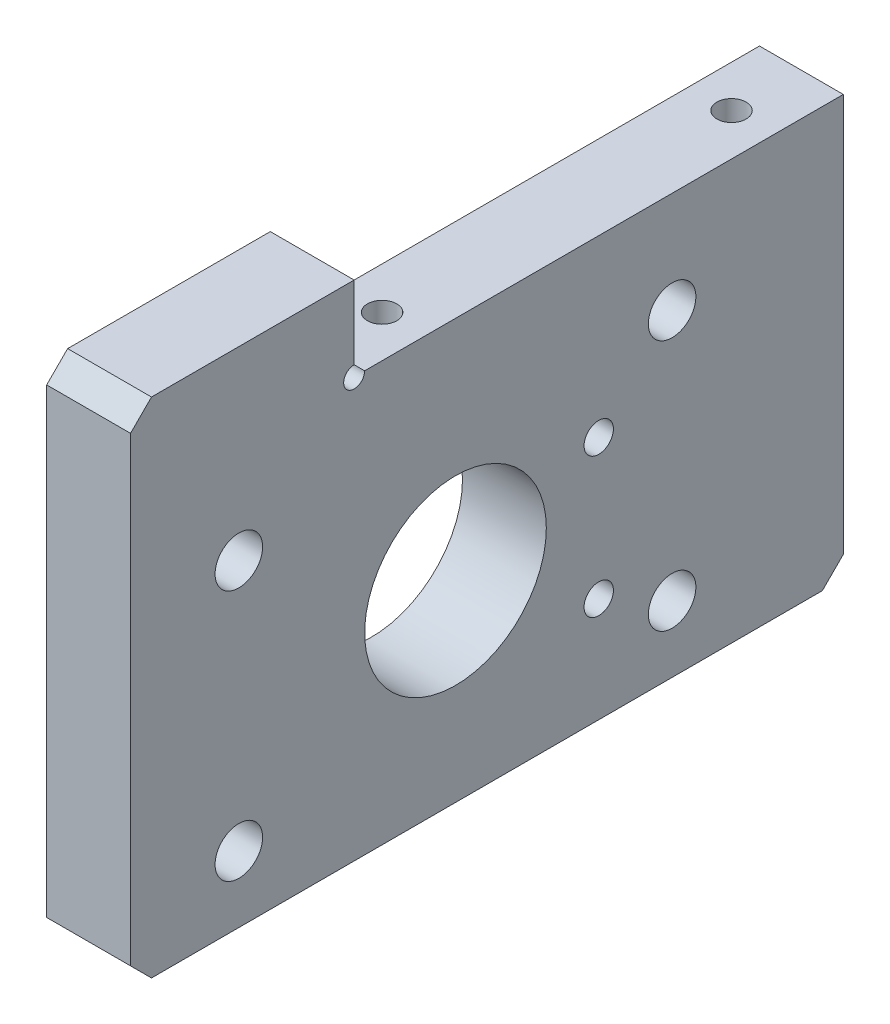
from build123d import *

# Parameters (mm, degrees)
BOSS_EXTRUDE1_DEPTH   = 12
SKETCH2_R             = 13
CUT_EXTRUDE1_DEPTH    = 126.427269762
M8_TAPPED_HOLE1_D     = 6.8
M8_TAPPED_HOLE1_DEPTH = 19.75
M8_TAPPED_HOLE1_TIP   = 2.042926105
M5_TAPPED_HOLE1_D     = 4.2
M5_TAPPED_HOLE1_DEPTH = 12.4
M5_TAPPED_HOLE1_TIP   = 1.2618073
M5_TAPPED_HOLE2_D     = 4.2
M5_TAPPED_HOLE2_DEPTH = 12.4
M5_TAPPED_HOLE2_TIP   = 1.2618073
CHAMFER1_SIZE         = 3
SKETCH11_R            = 1.5
CUT_EXTRUDE2_DEPTH    = 126.427269762


with BuildPart() as part:
    # Sketch1 → Boss-Extrude1 (new body)
    with BuildSketch(Plane(origin=(0, 0, 0), x_dir=(0, 0, -1), z_dir=(1, 0, 0))):
        Polygon((0, 0), (102, 0), (102, 60), (32, 60), (32, 72), (0, 72), align=None)
    extrude(amount=BOSS_EXTRUDE1_DEPTH)

    # Sketch2 → Cut-Extrude1 (cut, through all)
    with BuildSketch(Plane(origin=(12, 0, 0), x_dir=(0, 0, -1), z_dir=(1, 0, 0))):
        with Locations((46.5, 27.5)):
            Circle(SKETCH2_R)
    extrude(amount=-CUT_EXTRUDE1_DEPTH, mode=Mode.SUBTRACT)

    # M8 Tapped Hole1
    with Locations(Plane.ZY):
        with Locations((-77.5, 45.5), (-77.5, 9.5), (-15.5, 9.5), (-15.5, 45.5)):
            Hole(M8_TAPPED_HOLE1_D / 2, depth=M8_TAPPED_HOLE1_DEPTH)
            with Locations((0, 0, -(M8_TAPPED_HOLE1_DEPTH + M8_TAPPED_HOLE1_TIP / 2))):  # 118° drill point
                Cone(0, M8_TAPPED_HOLE1_D / 2, M8_TAPPED_HOLE1_TIP, mode=Mode.SUBTRACT)

    # M5 Tapped Hole1
    with Locations(Plane(origin=(12, 0, 0), x_dir=(0, 0, -1), z_dir=(1, 0, 0))):
        with Locations((67, 35), (67, 15)):
            Hole(M5_TAPPED_HOLE1_D / 2, depth=M5_TAPPED_HOLE1_DEPTH)
            with Locations((0, 0, -(M5_TAPPED_HOLE1_DEPTH + M5_TAPPED_HOLE1_TIP / 2))):  # 118° drill point
                Cone(0, M5_TAPPED_HOLE1_D / 2, M5_TAPPED_HOLE1_TIP, mode=Mode.SUBTRACT)

    # M5 Tapped Hole2
    with Locations(Plane(origin=(0, 60, 0), x_dir=(1, 0, 0), z_dir=(0, 1, 0))):
        with Locations((6, 42), (6, 92)):
            Hole(M5_TAPPED_HOLE2_D / 2, depth=M5_TAPPED_HOLE2_DEPTH)
            with Locations((0, 0, -(M5_TAPPED_HOLE2_DEPTH + M5_TAPPED_HOLE2_TIP / 2))):  # 118° drill point
                Cone(0, M5_TAPPED_HOLE2_D / 2, M5_TAPPED_HOLE2_TIP, mode=Mode.SUBTRACT)

    # Chamfer1
    chamfer1_edges = [part.edges().sort_by_distance(p)[0] for p in [
        (6, 72, 0),
        (6, 0, -102),
        (6, 0, 0),
    ]]
    chamfer(chamfer1_edges, length=CHAMFER1_SIZE)

    # Sketch11 → Cut-Extrude2 (cut, through all)
    with BuildSketch(Plane(origin=(12, 0, 0), x_dir=(0, 0, -1), z_dir=(1, 0, 0))):
        with Locations((32, 60)):
            Circle(SKETCH11_R)
    extrude(amount=-CUT_EXTRUDE2_DEPTH, mode=Mode.SUBTRACT)


solid = part.part
